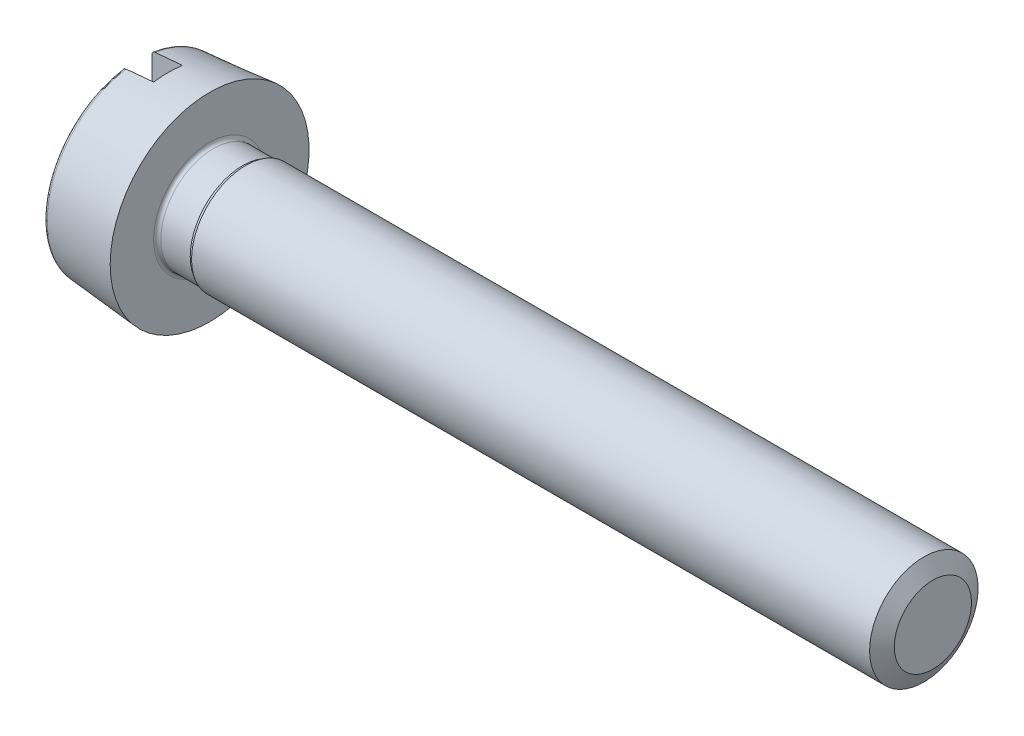
from build123d import *

# Parameters (mm, degrees)
CUT_EXTRUDE1_DEPTH = 0.85


with BuildPart() as part:
    # Sketch1 → Base-Revolve (revolve)
    with BuildSketch(Plane.XY, mode=Mode.PRIVATE) as base_revolve_sk:
        with BuildLine():
            Line((0, 0), (0, 2.483389556))
            ThreePointArc((0, 2.483389556), (0.026272266, 2.550948576), (0.091284426, 2.583009025))
            Line((0.091284426, 2.583009025), (2, 2.75))
            Line((2, 2.75), (2, 1.55))
            ThreePointArc((2, 1.55), (2.029289322, 1.479289322), (2.1, 1.45))
            Line((2.1, 1.45), (2.91339746, 1.45))
            Line((2.91339746, 1.45), (3, 1.5))
            Line((3, 1.5), (22, 1.5))
            Line((22, 1.5), (22, 0))
            Line((22, 0), (0, 0))
        make_face()
    revolve(base_revolve_sk.sketch.rotate(Axis((0, 0, 0), (1, 0, 0)), 90), axis=Axis((0, 0, 0), (1, 0, 0)))

    # Sketch2 → Cut-Extrude1 (cut)
    with BuildSketch(Plane.ZY):
        with BuildLine():
            Line((0.4, 2.720753572), (0.4, -2.720753572))
            ThreePointArc((0.4, -2.720753572), (0, -2.75), (-0.4, -2.720753572))
            Line((-0.4, -2.720753572), (-0.4, 2.720753572))
            ThreePointArc((-0.4, 2.720753572), (0, 2.75), (0.4, 2.720753572))
        make_face()
    extrude(amount=-CUT_EXTRUDE1_DEPTH, mode=Mode.SUBTRACT)

    # Sketch3 → Cut-Revolve1 (revolve, cut)
    with BuildSketch(Plane(origin=(0, 0, 0), x_dir=(1, 0, 0), z_dir=(0, 1, 0)), mode=Mode.PRIVATE) as cut_revolve1_sk:
        Polygon((21.750007333, 1.5), (22.249992667, 1.5), (22, 1.067), align=None)
    revolve(cut_revolve1_sk.sketch.rotate(Axis((0, 0, 0), (1, 0, 0)), 180), axis=Axis((0, 0, 0), (1, 0, 0)), mode=Mode.SUBTRACT)


solid = part.part
